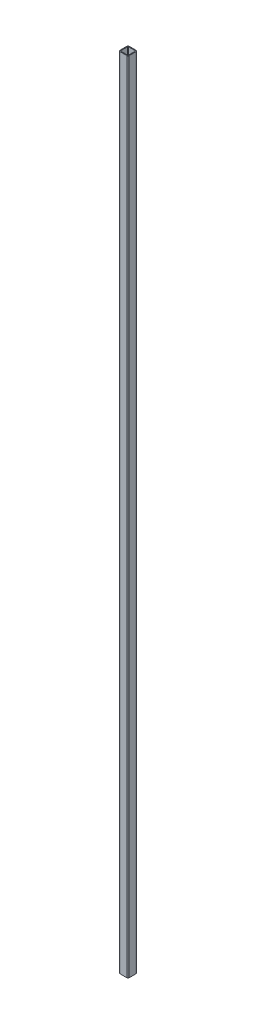
SolidWorks part; units mm, degrees
material "Q235B"
ref_plane "Front Plane" through (0, 0, 0) normal (0, 0, 1) x (1, 0, 0)
ref_plane "Top Plane" through (0, 0, 0) normal (0, 1, 0) x (1, 0, 0)
ref_plane "Right Plane" through (0, 0, 0) normal (1, 0, 0) x (0, 0, -1)
sketch "feature 17 (ProfileFeature) (+16 more in 12 files) Sketch1" plane through (0, 0, 0) normal (0, 0, 1) x (1, 0, 0)
  line L0 (0, 0) -> (0, 10370)
  dimension "D1" = 10370
other "Cold-formed Hollow Structural Square Steel(gb t6728-2002) 120×120×10(1)"
ref_plane "Plane1" through (0, 0, 0) normal (0, 1, 0) x (-1, 0, 0)
sketch "Sketch12" plane through (0, 0, 0) normal (0, 1, 0) x (-1, 0, 0)
  line L0 (-44, -50) -> (44, -50)
  line L1 (-50, -44) -> (-50, 44)
  line L2 (44, 50) -> (-44, 50)
  line L3 (50, 44) -> (50, -44)
  line L4 (-44, -60) -> (44, -60)
  line L5 (-60, -44) -> (-60, 44)
  line L6 (44, 60) -> (-44, 60)
  line L7 (60, 44) -> (60, -44)
  arc A0 (60, 44) -> (44, 60) centre (44, 44) ccw
  arc A1 (44, -60) -> (60, -44) centre (44, -44) ccw
  arc A2 (-60, -44) -> (-44, -60) centre (-44, -44) ccw
  arc A3 (-44, 60) -> (-60, 44) centre (-44, 44) ccw
  arc A4 (-44, 50) -> (-50, 44) centre (-44, 44) ccw
  arc A5 (50, 44) -> (44, 50) centre (44, 44) ccw
  arc A6 (44, -50) -> (50, -44) centre (44, -44) ccw
  arc A7 (-50, -44) -> (-44, -50) centre (-44, -44) ccw
  point P0 (-60, 0)
  point P1 (60, 0)
  point P2 (0, 60)
  point P3 (0, -60)
  point P4 (0, 0)
  point P5 (-60, -60)
  point P6 (60, -60)
  point P7 (60, 60)
  point P8 (-60, 60)
  point P33 (0, 0)
  dimension "D1" = 16
  dimension "D2" = 120
  dimension "D3" = 10
